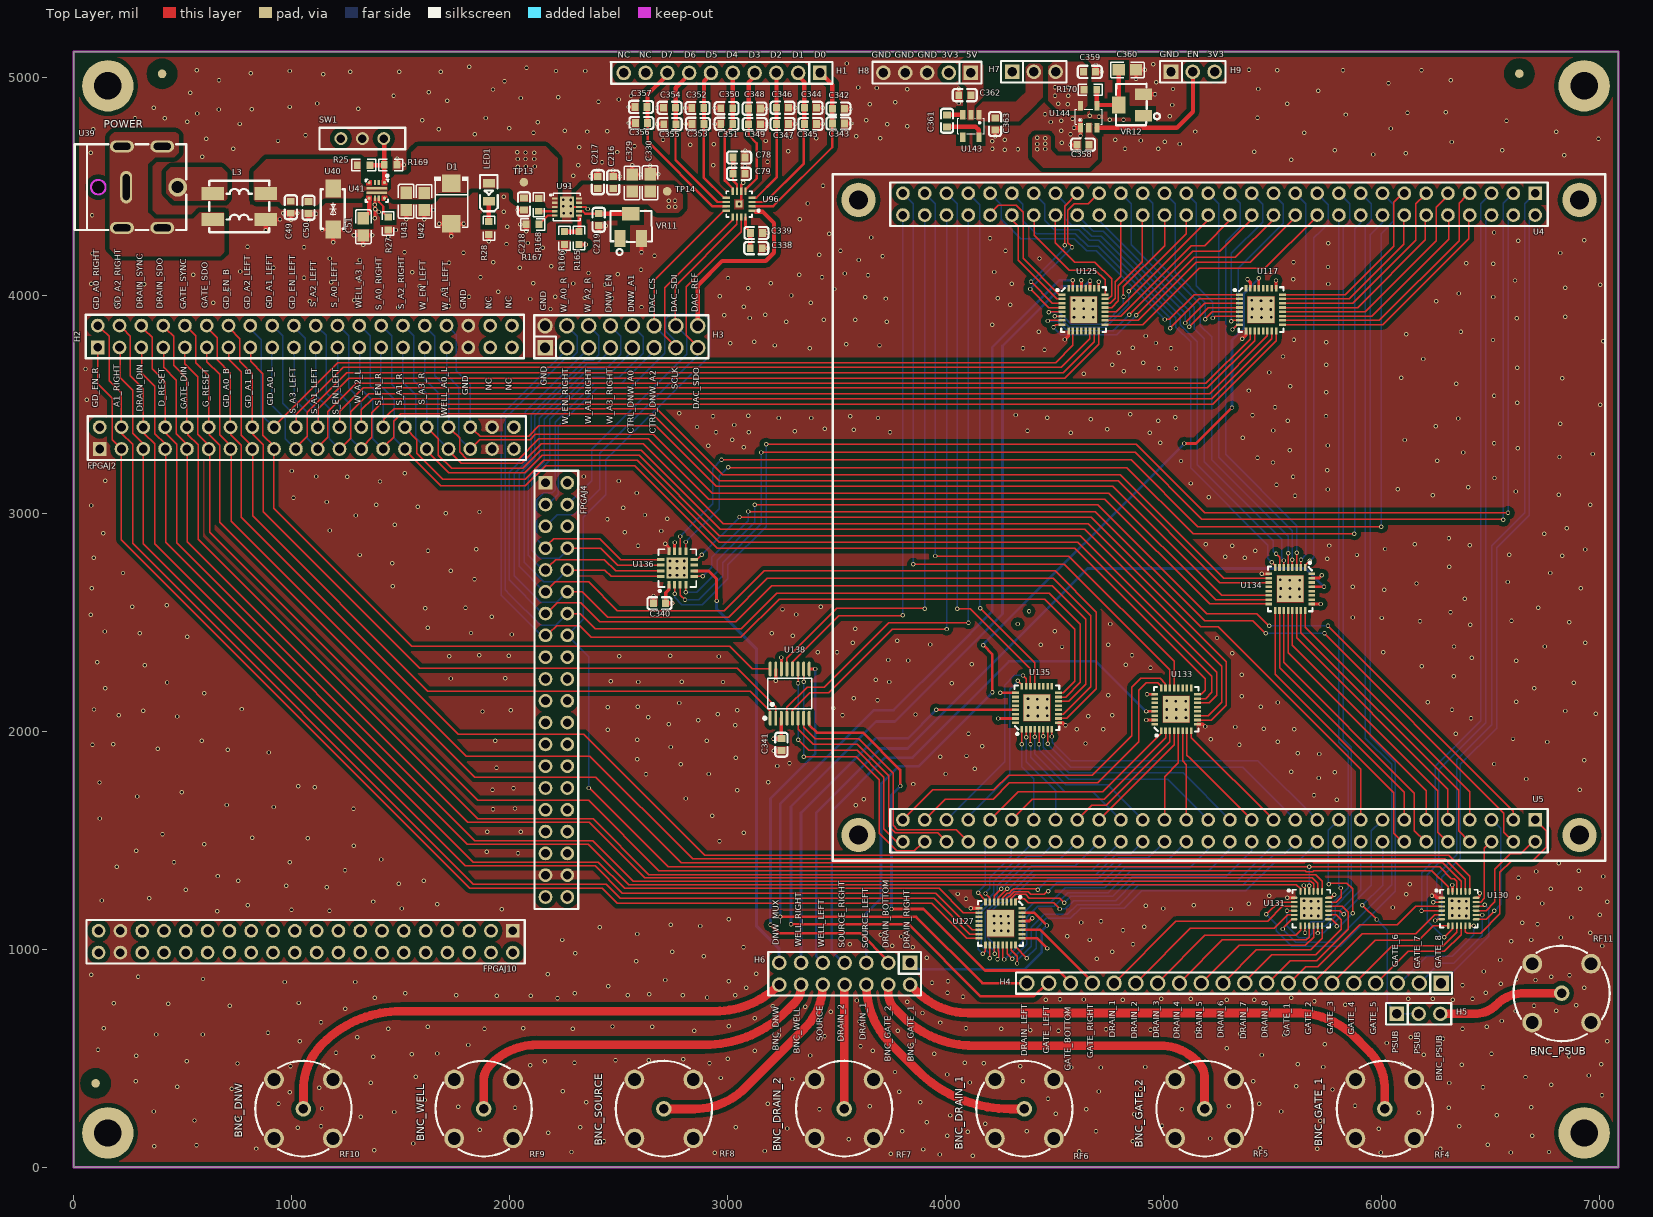
[diagram p0: Top Layer view]
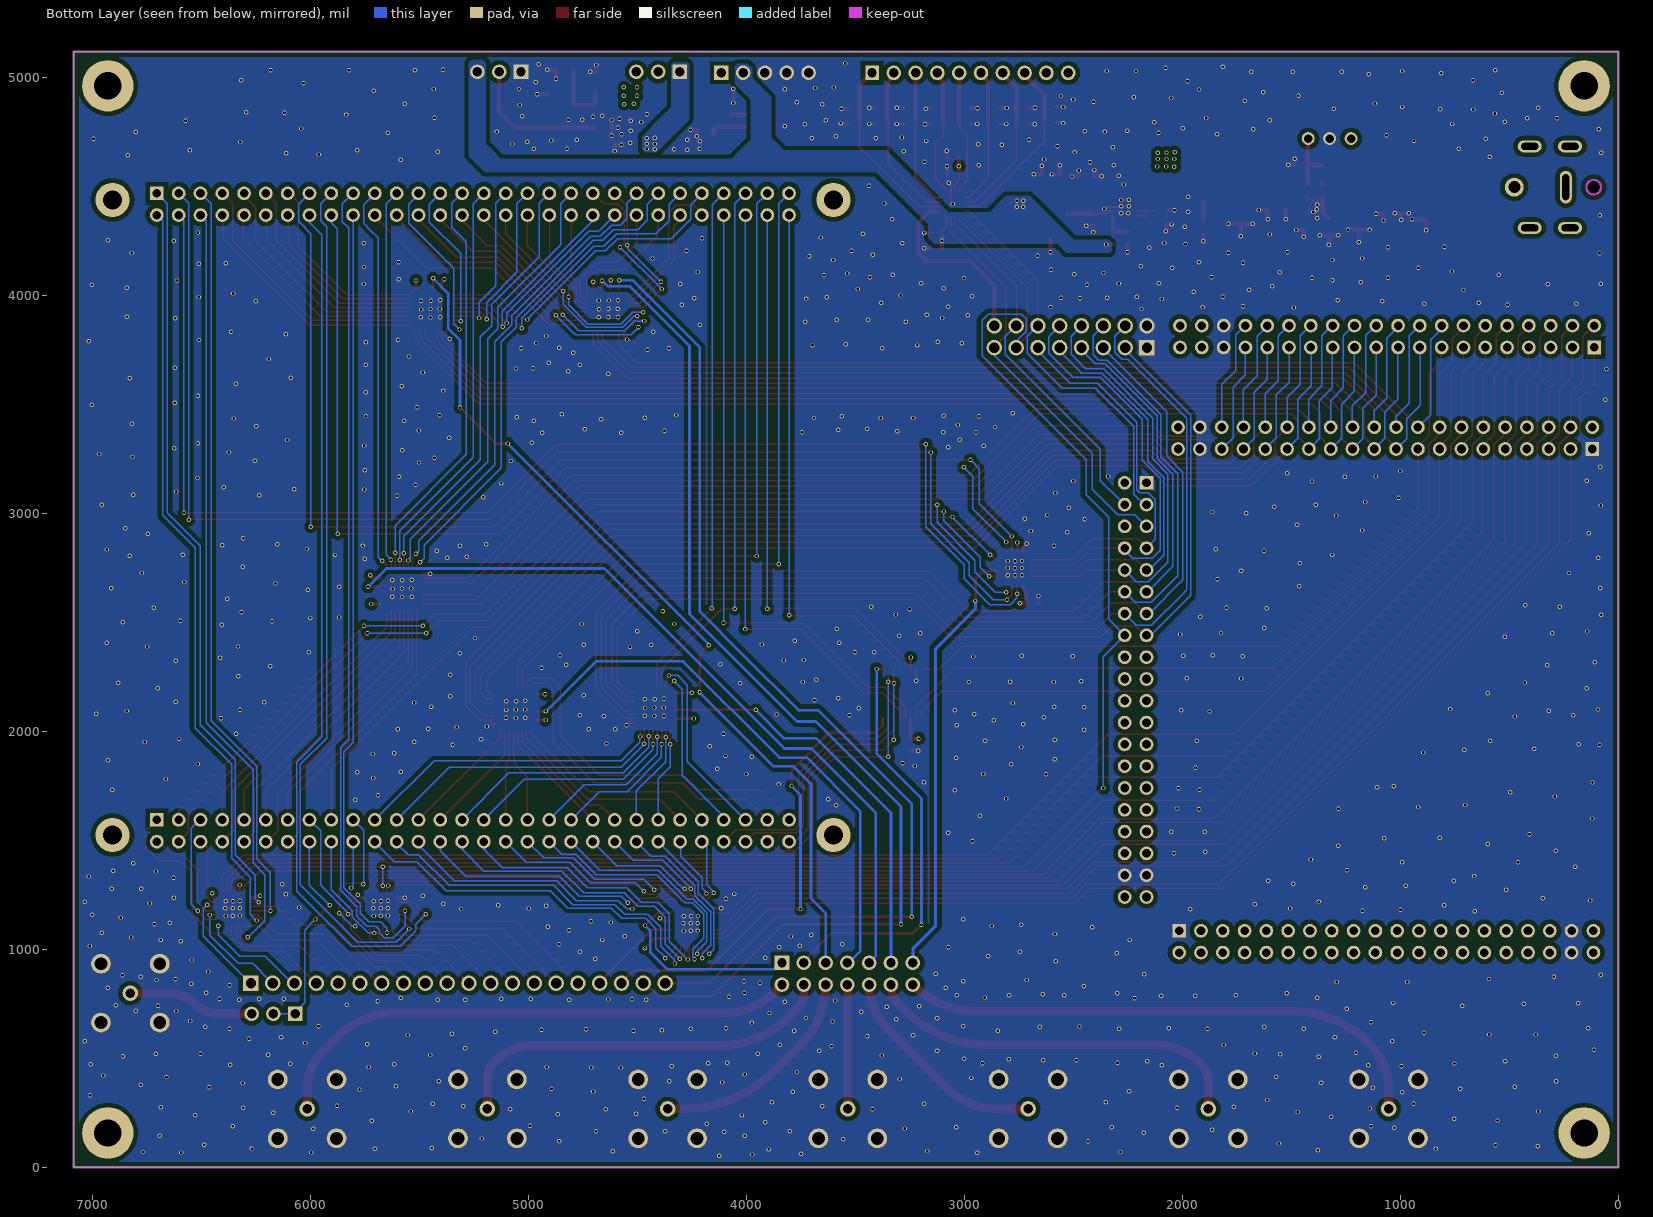
[diagram p1: Bottom Layer view, seen from below]
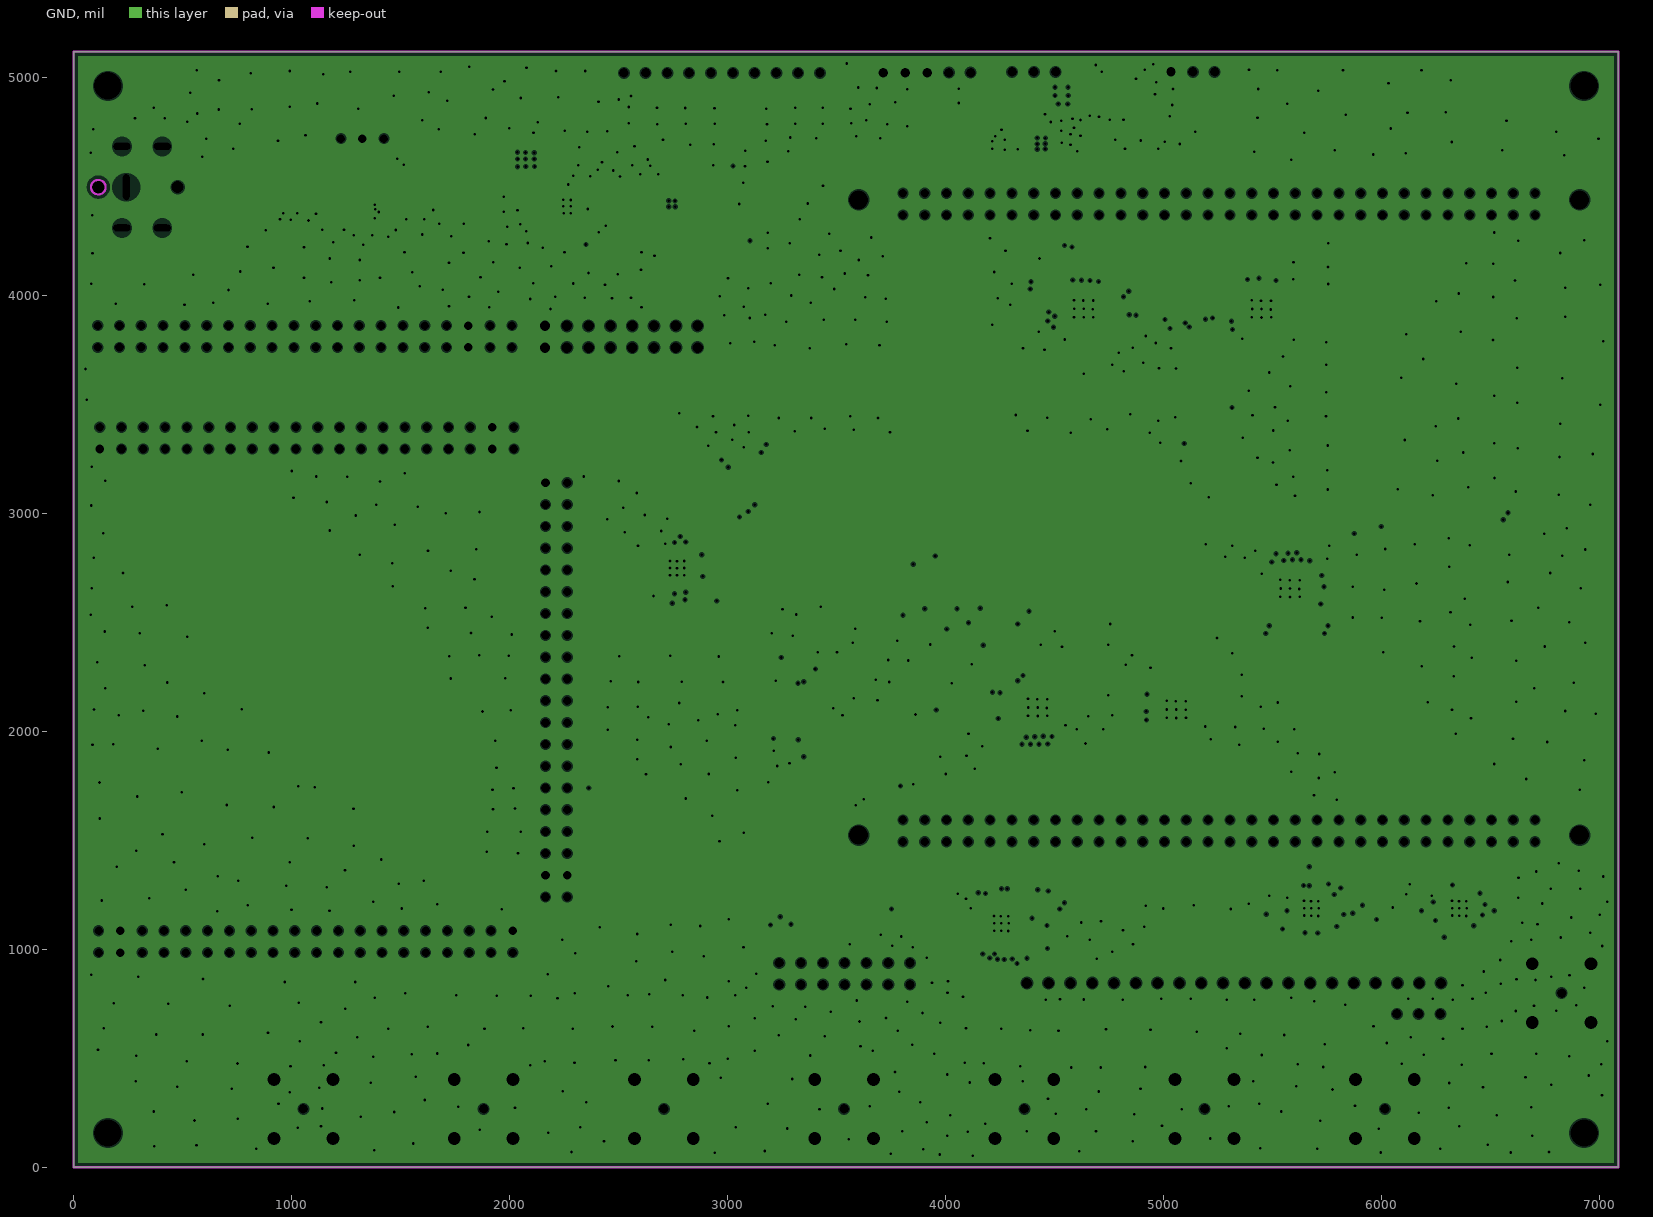
[diagram p2: GND, clearances drawn from the general rule]
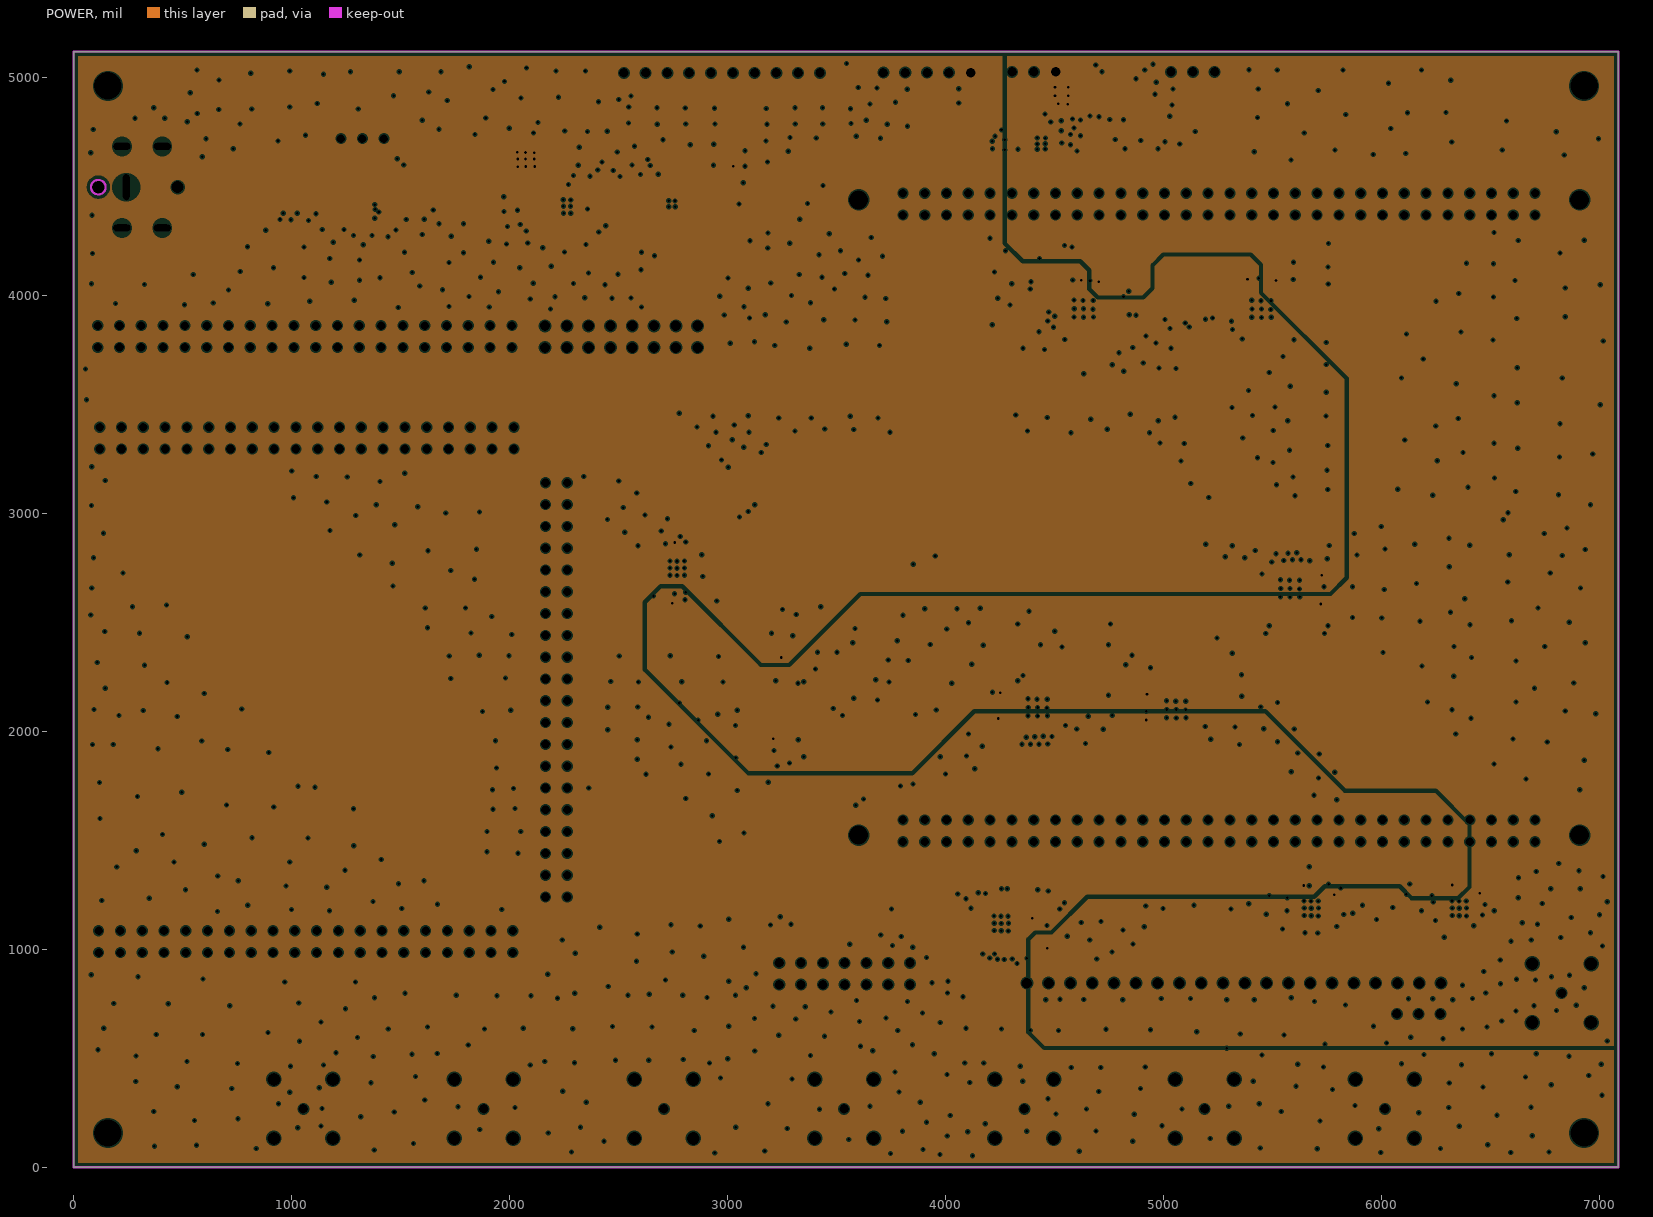
[diagram p3: POWER, clearances drawn from the general rule]
# Altium PCB MISC82799.PcbDoc (part 1 of 5)
Units mil, origin at the board's own origin, x right, y up, seen from the top; angles counter-clockwise.
Board outline 7086.61 x 5118.11 mil, 4 copper layers (Top Layer, GND, POWER, Bottom Layer); 95 components, 232 nets, 857 pads, 1291 vias.

## Layer stack, top to bottom (the 12.6 mil dielectric is the usual default, probably not edited)
Top Layer: signal copper 1.4
Dielectric: core 12.6, FR-4, Dk 4.8
GND: plane copper 1.4, net GND
Dielectric: prepreg 12.6, FR-4, Dk 4.8
POWER: plane copper 1.4, net (Multiple Nets)
Dielectric: core 12.6, FR-4, Dk 4.8
Bottom Layer: signal copper 1.4

## Board outline
0,0 7086.61,0 7086.61,5118.11 0,5118.11

## Design rules (kind name [scope] priority, off if disabled: settings)
Clearance Clearance_2 [haspad('free-mark')] p1: gap=50
Clearance Clearance_1 [inpolygon] p2: gap=6
Clearance [All] p3: gap=6
DiffPairsRouting [All] p1: maxlimit=6 minlimit=6 mostfreqgap=6 maxuncoupledlength=500
HoleSize [All] p1: absolutevalues=TRUE maxlimit=500 minlimit=1 maxpercent=80.000 minpercent=20.000
HoleToHoleClearance [All] p1: gap=0 allowstackedmicrovias=TRUE
MinimumSolderMaskSliver [All] p1: minsoldermaskwidth=0
PlaneClearance [All] p1: clearance=6
PlaneConnect [All] p1: planeconnectstyle=Direct reliefexpansion=20 reliefentries=4 reliefconductorwidth=10 reliefairgap=10
PolygonConnect [All] p1: connectstyle=Direct reliefconductorwidth=10 reliefentries=4 polygonreliefangle="90 Angle"
RoutingVias [All] p1: holewidth=12 width=20 viastyle="Through Hole" minholewidth=12 minwidth=20 maxholewidth=12 maxwidth=20
SilkToSilkClearance [All] p1: silktosilkclearance=0
SilkscreenOverComponentPads [All] p1: minsilkscreentomaskgap=0
SolderMaskExpansion [All] p1: expansion=4
Width [All] p1: maxlimit=40 minlimit=6 preferedwidth=6
20 further rules are at their usual default settings.

## Classes and differential pairs
component class 2_MUX: H4 H5 H6 RF4 RF5 RF6 RF7 RF8 RF9 RF10 RF11 U117 U125 U127 U130 U131 U133 U134 U135 U136 U138
component class 1_Power: C49 C50 C51 C78 C79 C216 C217 C218 C219 C329 C330 C338 C339 C340 C341 C342 C343 C344 C345 C346 C347 C348 C349 C350 C351 C352 C353 C354 C355 C356 C357 C358 C359 C360 C361 C362 C363 D1 FPGAJ2 FPGAJ4 FPGAJ10 H1 H2 H3 H7 H8 H9 L3 LED1 R25 R27 R28 R165 R166 R167 R168 R169 R170 SW1 TP13 TP14 U4 U5 U39 U40 U41 U42 U43 U91 U96 U143 U144 VR11 VR12

## Components (designator, comment, footprint, x,y, rotation, side; value= is the part's Value field where it differs from the comment)
C49 "100nF" C0603 997,4404 r90 top
C50 "100nF" C0603 1078,4402 r90 top
C51 "10nF" C0805 1329,4314 r90 top
C78 "100nF" C0603 3053,4632 r180 top
C79 "10uF" C0603 3052.24,4557.36 r180 top
C216 "22uF" C0603 2475.61,4517.13 r270 top
C217 "22uF" C0603 2405,4518 r270 top
C218 "22uF" C0603 2066,4418 r90 top
C219 "4.7uF" C0603 2409,4347 r90 top
C329 "100nF" C0805 2562.12,4515 r270 top
C330 "10uF" C0805 2645,4516 r270 top
C338 "100nF" C0603 3131.5,4216.36 r180 top
C339 "10uF" C0603 3132,4286 r180 top
C340 "100nF" C0603 2688,2587 r0 top
C341 "10uF" C0603 3247,1939 r90 top
C342 "100nF" C0603 3508.15,4856 r180 top
C343 "10uF" C0603 3508.39,4788.31 r180 top
C344 "100nF" C0603 3380.15,4860 r180 top
C345 "10uF" C0603 3380.15,4786 r180 top
C346 "100nF" C0603 3252.16,4860.31 r180 top
C347 "10uF" C0603 3252.15,4786 r180 top
C348 "100nF" C0603 3123.67,4856.31 r180 top
C349 "10uF" C0603 3124.15,4785 r180 top
C350 "100nF" C0603 2996.15,4858 r0 top
C351 "10uF" C0603 2996.15,4786 r0 top
C352 "100nF" C0603 2863.15,4859 r0 top
C353 "10uF" C0603 2864.15,4786 r0 top
C354 "100nF" C0603 2734.15,4859.89 r0 top
C355 "10uF" C0603 2735.15,4785 r0 top
C356 "100nF" C0603 2605.15,4790 r0 top
C357 "10uF" C0603 2603.39,4863.89 r0 top
C358 "2.2uF" C0603 4631,4691 r0 top
C359 "2.2uF" C0603 4661,5025 r180 top
C360 "10nF" C0805 4834,5034 r180 top
C361 "1uF" C0603 4006.33,4800.13 r270 top
C362 "1uF" C0603 4088.33,4918.13 r0 top
C363 "1uF" C0603 4227.33,4786.13 r90 top
D1 "VS-10BQ015HM3/5BT" SMB_L4.6-W3.6-LS5.3-RD 1733,4421 r270 top
FPGAJ2 "2.54-2*20" HDR-TH_40P-P2.54-V-F-R2-C20-S2.54 1070,3345 r0 top
FPGAJ4 "2.54-2*20" HDR-TH_40P-P2.54-V-F-R2-C20-S2.54 2215,2190 r270 top
FPGAJ10 "2.54-2*20" HDR-TH_40P-P2.54-V-F-R2-C20-S2.54 1065,1035 r180 top
H1 "PZ254V-11-10P" HDR-TH_10P-P2.54-V-M 2974,5020 r180 top
H2 "PZ254-2-20-W-8.5" HDR-TH_40P-P2.54-V-F-R2-C20-S2.54 1061,3811 r0 top
H3 "PZ254V-12-16P" HDR-TH_16P-P2.54-V-M-R2-C8-S2.54 2513,3810 r0 top
H4 "PZ254-1-20-W-8.5" HDR-TH_20P-P2.54-V-M-1 5323,845 r180 top
H5 "PZ254V-11-03P" HDR-TH_3P-P2.54-V-M 6170,704 r0 top
H6 "PZ254V-12-14P" HDR-TH_14P-P2.54-V-M-R2-C7-S2.54 3537,888 r180 top
H7 "PZ254V-11-03P" HDR-TH_3P-P2.54-V-M 4405,5025 r0 top
H8 "PZ254V-11-05P" HDR-TH_5P-P2.54-V-M 3915,5021 r180 top
H9 "PZ254V-11-03P" HDR-TH_3P-P2.54-V-M 5134,5025 r0 top
L3 "PCAQ7060MW-301" FILTER-SMD_4P-L7.0-W6.0-BL 760,4407 r270 top
LED1 "NCD0805G1" LED0805-R-RD 1905,4473 r90 top
R25 "" R0603 1331,4597 r0 top
R27 "" R0603 1443,4329 r270 top
R28 "" R0603 1905,4308 r90 top
R165 "" R0603 2318.61,4262.42 r270 top
R166 "" R0603 2252,4262 r90 top
R167 "" R0603 2106,4325 r0 top
R168 "" R0603 2134,4415 r90 top
R169 "" R0603 1455,4598 r0 top
R170 "" R0603 4664,4943 r180 top
RF4 "DOSIN-801-0057" ANT-TH_DOSIN-801-0057 6015,268 r180 top
RF5 "DOSIN-801-0057" ANT-TH_DOSIN-801-0057 5188.23,268 r180 top
RF6 "DOSIN-801-0057" ANT-TH_DOSIN-801-0057 4361.46,268 r180 top
RF7 "DOSIN-801-0057" ANT-TH_DOSIN-801-0057 3534.68,268 r180 top
RF8 "DOSIN-801-0057" ANT-TH_DOSIN-801-0057 2707.91,268 r180 top
RF9 "DOSIN-801-0057" ANT-TH_DOSIN-801-0057 1881.14,268 r180 top
RF10 "DOSIN-801-0057" ANT-TH_DOSIN-801-0057 1054.37,268 r180 top
RF11 "DOSIN-801-0057" ANT-TH_DOSIN-801-0057 6826,799 r0 top
SW1 "K3-1204D" SW-TH_K3-1204D 1325,4719 r0 top
TP13 "5V" Test-Point-0.5mm 2066,4519 r90 top
TP14 "3P3V" Test-Point-0.5mm 2723,4477 r90 top
U4 "ZX-PM2.54-2-30PY" HDR-TH_60P-P2.54-V-F-R2-C30-S2.54 5254.35,4417.81 r180 top locked
U5 "ZX-PM2.54-2-30PY" HDR-TH_60P-P2.54-V-F-R2-C30-S2.54 5254.35,1543.8 r180 top locked
U39 "HX DC007B-2.5" DC-IN-TH_HX-DC007B-2.5 350,4496 r0 top
U40 "SMAJ12CA" SMA_L4.3-W2.7-LS5.1-BI 1191,4396 r90 top
U41 "TPS259472ARPWR" VQFN-10_L2.0-W2.0-P0.45-TL 1391,4481 r270 top
U42 "22uF" C0805 1608.25,4430.56 r90 top
U43 "22uF" C0805 1526,4431 r90 top
U91 "LT3045IDD#PBF" DFN-10_L3.0-W3.0-P0.50-BL-EP-3 2263,4405 r270 top
U96 "DAC80508ZRTER" WQFN-16_L3.0-W3.0-P0.50-TL-EP0.8 3053,4418 r180 top
U117 "ADG1406BCPZ-REEL7" LFCSP-32_L5.0-W5.0-P0.50-TL-EP3.1 5447,3934 r0 top
U125 "ADG1407BCPZ-REEL7" LFCSP-32_L5.0-W5.0-P0.50-BL-EP3.1 4633,3934 r270 top locked
U127 "ADG1407BCPZ-REEL7" LFCSP-32_L5.0-W5.0-P0.50-BL-EP3.1 4252,1119 r180 top
U130 "ADG1414BCPZ-REEL7" LFCSP-24_L4.0-W4.0-P0.50-BL-EP 6355,1187 r270 top locked
U131 "ADG1414BCPZ-REEL7" LFCSP-24_L4.0-W4.0-P0.50-BL-EP 5678,1187 r270 top
U133 "ADG1406BCPZ-REEL7" LFCSP-32_L5.0-W5.0-P0.50-TL-EP3.1 5058,2101 r90 top
U134 "ADG1406BCPZ-REEL7" LFCSP-32_L5.0-W5.0-P0.50-TL-EP3.1 5581,2653 r270 top
U135 "ADG1406BCPZ-REEL7" LFCSP-32_L5.0-W5.0-P0.50-TL-EP3.1 4419,2108 r90 top
U136 "ADG1408YCPZ-REEL7" LFCSP-16_L4.0-W4.0-P0.65-BL-EP 2770,2749 r0 top
U138 "ADG1409YRUZ-REEL7" TSSOP-16_L5.0-W4.4-P0.65-LS6.4-BL 3285,2173 r0 top
U143 "TPS60403DBVR" SOT-23-5_L3.0-W1.7-P0.95-LS2.8-BR 4116.12,4776.13 r90 top
U144 "TPS72301DBVR" SOT-23-5_L3.0-W1.7-P0.95-LS2.8-BR 4656.56,4819 r270 top
VR11 "" RES-ADJ-SMD_3224W 2556,4317 r0 top
VR12 "" RES-ADJ-SMD_3224W 4851,4873 r90 top

## Footprints (in the part's own frame and the unit in brackets; to place one, negate y for a bottom-side part, rotate by r counter-clockwise, add the part's x,y. Pads: shape width x height; smd on the part's side, far side on the other; paste and mask are expansions set on the pad)
ANT-TH_DOSIN-801-0057 [mm]
  round 1.8 hole 1.1: 1(0,0)
  round 2.3 hole 1.5: 2(-3.429,3.429) 3(3.429,3.429) 4(3.429,-3.429) 5(-3.429,-3.429)
  silkscreen extent -5.6,-5.6 5.6,5.53
C0603 [mm]
  rect 0.8x0.9 smd: 1(-0.7,0) 2(0.7,0)
  silkscreen extent -1.41,-0.71 1.39,0.72
C0805 [mm]
  rect 1.41x1.35 smd paste-100 mask+0.051: 1(-1,0) 2(1,0)
  silkscreen extent -1.96,-0.9 1.96,0.9
DC-IN-TH_HX-DC007B-2.5 [mm]
  round 2.2 hole 1.4: 1(3.25,0)
  oval 1.4x3.8 hole 0.8 slot 3 at 90 deg: 2(-2.75,0)
  oval 2.8x1.4 hole 0.8 slot 2 at 0 deg: 3(-3.25,-4.75) 3(-3.25,4.75) 3(1.45,-4.75) 3(1.45,4.75)
  Keep-Out Layer circle w0.005: c-6,0 r0.85
  Keep-Out Layer board cut-out: -5.15,0 -5.234,0.369 -5.47,0.664 -5.811,0.829 -6.189,0.829 -6.53,0.664 -6.766,0.369 -6.85,0 -6.85,0 -6.766,-0.369 -6.53,-0.665 -6.189,-0.829 -5.811,-0.829 -5.47,-0.665 -5.234,-0.369 -5.15,0
  Keep-Out Layer circle w0.254: c-6,0 r0.85
  silkscreen extent -8.75,-5 4.25,5
DFN-10_L3.0-W3.0-P0.50-BL-EP-3 [mm]
  rect 0.25x0.65 smd: 1(-1,-1.411) 2(-0.5,-1.411) 3(0,-1.411) 4(0.5,-1.411) 5(1,-1.411) 6(1,1.411) 7(0.5,1.411) 8(0,1.411) 9(-0.5,1.411) 10(-1,1.411)
  rect 2.5x1.6 smd: 11(0,0)
  silkscreen extent -1.58,-2 1.58,1.58
FILTER-SMD_4P-L7.0-W6.0-BL [mm]
  rect 1.501x2.6 smd: 1(-1.5,-3.1) 2(1.5,-3.1) 3(1.5,3.1) 4(-1.5,3.1)
  silkscreen extent -3,-3.5 3,3.5
HDR-TH_3P-P2.54-V-M [mm]
  rect 1.7x1.7 hole 1.1: 1(-2.54,0)
  round 1.7 hole 1.1: 2(0,0) 3(2.54,0)
  silkscreen extent -3.81,-1.25 3.81,1.25
HDR-TH_5P-P2.54-V-M [mm]
  rect 1.7x1.7 hole 1.1: 1(-5.08,0)
  round 1.7 hole 1.1: 2(-2.54,0) 3(0,0) 4(2.54,0) 5(5.08,0)
  silkscreen extent -6.35,-1.27 6.35,1.27
HDR-TH_10P-P2.54-V-M [mm]
  rect 1.575x1.7 hole 1.1: 1(-11.43,0)
  round 1.7 hole 1.1: 2(-8.89,0) 3(-6.35,0) 4(-3.81,0) 5(-1.27,0) 6(1.27,0) 7(3.81,0) 8(6.35,0) 9(8.89,0) 10(11.43,0)
  silkscreen extent -12.9,-1.27 12.95,1.27
HDR-TH_14P-P2.54-V-M-R2-C7-S2.54 [mm]
  rect 1.7x1.7 hole 1.1: 1(-7.62,-1.27)
  round 1.7 hole 1.1: 2(-7.62,1.27) 3(-5.08,-1.27) 4(-5.08,1.27) 5(-2.54,-1.27) 6(-2.54,1.27) 7(0,-1.27) 8(0,1.27) 9(2.54,-1.27) 10(2.54,1.27) 11(5.08,-1.27) 12(5.08,1.27) 13(7.62,-1.27) 14(7.62,1.27)
  silkscreen extent -8.89,-2.54 8.89,2.54
HDR-TH_16P-P2.54-V-M-R2-C8-S2.54 [mm]
  rect 1.8x1.8 hole 1.2: 1(-8.89,-1.27)
  round 1.8 hole 1.2: 2(-8.89,1.27) 3(-6.35,-1.27) 4(-6.35,1.27) 5(-3.81,-1.27) 6(-3.81,1.27) 7(-1.27,-1.27) 8(-1.27,1.27) 9(1.27,-1.27) 10(1.27,1.27) 11(3.81,-1.27) 12(3.81,1.27) 13(6.35,-1.27) 14(6.35,1.27) 15(8.89,-1.27) 16(8.89,1.27)
  silkscreen extent -10.16,-2.5 10.16,2.5
HDR-TH_20P-P2.54-V-M-1 [mm]
  rect 1.8x1.8 hole 1.2: 1(-24.13,0)
  round 1.8 hole 1.2: 2(-21.59,0) 3(-19.05,0) 4(-16.51,0) 5(-13.97,0) 6(-11.43,0) 7(-8.89,0) 8(-6.35,0) 9(-3.81,0) 10(-1.27,0) 11(1.27,0) 12(3.81,0) 13(6.35,0) 14(8.89,0) 15(11.43,0) 16(13.97,0) 17(16.51,0) 18(19.05,0) 19(21.59,0) 20(24.13,0)
  silkscreen extent -25.4,-1.25 25.4,1.25
HDR-TH_40P-P2.54-V-F-R2-C20-S2.54 [mm]
  rect 1.6x1.6 hole 1: 1(-24.13,-1.27)
  round 1.6 hole 1: 2(-24.13,1.27) 3(-21.59,-1.27) 4(-21.59,1.27) 5(-19.05,-1.27) 6(-19.05,1.27) 7(-16.51,-1.27) 8(-16.51,1.27) 9(-13.97,-1.27) 10(-13.97,1.27) 11(-11.43,-1.27) 12(-11.43,1.27) 13(-8.89,-1.27) 14(-8.89,1.27) 15(-6.35,-1.27) 16(-6.35,1.27) 17(-3.81,-1.27) 18(-3.81,1.27) 19(-1.27,-1.27) 20(-1.27,1.27) 21(1.27,-1.27) 22(1.27,1.27) 23(3.81,-1.27) 24(3.81,1.27) 25(6.35,-1.27) 26(6.35,1.27) 27(8.89,-1.27) 28(8.89,1.27) 29(11.43,-1.27) 30(11.43,1.27) 31(13.97,-1.27) 32(13.97,1.27) 33(16.51,-1.27) 34(16.51,1.27) 35(19.05,-1.27) 36(19.05,1.27) 37(21.59,-1.27) 38(21.59,1.27) 39(24.13,-1.27) 40(24.13,1.27)
  silkscreen extent -25.53,-2.54 25.53,2.54
HDR-TH_60P-P2.54-V-F-R2-C30-S2.54 [mm]
  rect 1.6x1.6 hole 1: 1(-36.83,-1.27)
  round 1.6 hole 1: 2(-36.83,1.27) 3(-34.29,-1.27) 4(-34.29,1.27) 5(-31.75,-1.27) 6(-31.75,1.27) 7(-29.21,-1.27) 8(-29.21,1.27) 9(-26.67,-1.27) 10(-26.67,1.27) 11(-24.13,-1.27) 12(-24.13,1.27) 13(-21.59,-1.27) 14(-21.59,1.27) 15(-19.05,-1.27) 16(-19.05,1.27) 17(-16.51,-1.27) 18(-16.51,1.27) 19(-13.97,-1.27) 20(-13.97,1.27) 21(-11.43,-1.27) 22(-11.43,1.27) 23(-8.89,-1.27) 24(-8.89,1.27) 25(-6.35,-1.27) 26(-6.35,1.27) 27(-3.81,-1.27) 28(-3.81,1.27) 29(-1.27,-1.27) 30(-1.27,1.27) 31(1.27,-1.27) 32(1.27,1.27) 33(3.81,-1.27) 34(3.81,1.27) 35(6.35,-1.27) 36(6.35,1.27) 37(8.89,-1.27) 38(8.89,1.27) 39(11.43,-1.27) 40(11.43,1.27) 41(13.97,-1.27) 42(13.97,1.27) 43(16.51,-1.27) 44(16.51,1.27) 45(19.05,-1.27) 46(19.05,1.27) 47(21.59,-1.27) 48(21.59,1.27) 49(24.13,-1.27) 50(24.13,1.27) 51(26.67,-1.27) 52(26.67,1.27) 53(29.21,-1.27) 54(29.21,1.27) 55(31.75,-1.27) 56(31.75,1.27) 57(34.29,-1.27) 58(34.29,1.27) 59(36.83,-1.27) 60(36.83,1.27)
  silkscreen extent -38.3,-2.54 38.3,2.54
LED0805-R-RD [mm]
  rect 1x1.4 smd: 1(1.05,0) 2(-1.05,0)
  silkscreen extent -2.22,-1.04 1.99,1.01
LFCSP-16_L4.0-W4.0-P0.65-BL-EP [mm]
  rect 0.35x0.9 smd: 1(-0.975,-1.95) 2(-0.325,-1.95) 3(0.325,-1.95) 4(0.975,-1.95) 9(0.975,1.95) 10(0.325,1.95) 11(-0.325,1.95) 12(-0.975,1.95)
  rect 0.9x0.35 smd: 5(1.95,-0.975) 6(1.95,-0.325) 7(1.95,0.325) 8(1.95,0.975) 13(-1.95,0.975) 14(-1.95,0.325) 15(-1.95,-0.325) 16(-1.95,-0.975)
  rect 2.5x2.5 smd: 17(0,0)
  silkscreen extent -2.2,-2.8 2.2,2.2
LFCSP-24_L4.0-W4.0-P0.50-BL-EP [mm]
  oval 0.25x0.8 smd paste-100 mask+0.051: 1(-1.25,-2) 2(-0.749,-2) 3(-0.249,-2) 4(0.249,-2) 5(0.749,-2) 6(1.25,-2) 13(1.25,2) 14(0.749,2) 15(0.249,2) 16(-0.249,2) 17(-0.749,2) 18(-1.25,2)
  oval 0.8x0.25 smd paste-100 mask+0.051: 7(2,-1.25) 8(2,-0.749) 9(2,-0.249) 10(2,0.249) 11(2,0.749) 12(2,1.25) 19(-2,1.25) 20(-2,0.749) 21(-2,0.249) 22(-2,-0.249) 23(-2,-0.749) 24(-2,-1.25)
  rect 2.6x2.6 smd paste-100 mask+0.051: 25(0,0)
  silkscreen extent -2.22,-2.75 2.2,2.2
LFCSP-32_L5.0-W5.0-P0.50-BL-EP3.1 [mm]
  rect 0.3x0.8 smd paste-100 mask+0.051: 1(-1.75,-2.5) 2(-1.25,-2.5) 3(-0.75,-2.5) 4(-0.25,-2.5) 5(0.25,-2.5) 6(0.75,-2.5) 7(1.25,-2.5) 8(1.75,-2.5) 17(1.75,2.5) 18(1.25,2.5) 19(0.75,2.5) 20(0.25,2.5) 21(-0.25,2.5) 22(-0.75,2.5) 23(-1.25,2.5) 24(-1.75,2.5)
  rect 0.8x0.3 smd paste-100 mask+0.051: 9(2.5,-1.75) 10(2.5,-1.25) 11(2.5,-0.75) 12(2.5,-0.25) 13(2.5,0.25) 14(2.5,0.75) 15(2.5,1.25) 16(2.5,1.75) 25(-2.5,1.75) 26(-2.5,1.25) 27(-2.5,0.75) 28(-2.5,0.25) 29(-2.5,-0.25) 30(-2.5,-0.75) 31(-2.5,-1.25) 32(-2.5,-1.75)
  rect 3.1x3.1 smd paste-100 mask+0.051: 33(0,0)
  silkscreen extent -2.6,-3.17 2.6,2.6
LFCSP-32_L5.0-W5.0-P0.50-TL-EP3.1 [mm]
  rect 0.8x0.3 smd paste-100 mask+0.05: 1(-2.5,1.75) 2(-2.5,1.25) 3(-2.5,0.75) 4(-2.5,0.25) 5(-2.5,-0.25) 6(-2.5,-0.75) 7(-2.5,-1.25) 8(-2.5,-1.75) 17(2.5,-1.75) 18(2.5,-1.25) 19(2.5,-0.75) 20(2.5,-0.25) 21(2.5,0.25) 22(2.5,0.75) 23(2.5,1.25) 24(2.5,1.75)
  rect 0.3x0.8 smd paste-100 mask+0.05: 9(-1.75,-2.5) 10(-1.25,-2.5) 11(-0.75,-2.5) 12(-0.25,-2.5) 13(0.25,-2.5) 14(0.75,-2.5) 15(1.25,-2.5) 16(1.75,-2.5) 25(1.75,2.5) 26(1.25,2.5) 27(0.75,2.5) 28(0.25,2.5) 29(-0.25,2.5) 30(-0.75,2.5) 31(-1.25,2.5) 32(-1.75,2.5)
  rect 3.1x3.1 smd paste-100 mask+0.05: 33(0,0)
  silkscreen extent -3.17,-2.6 2.6,2.6
R0603 [mil]
  rect 31.75x34.02 smd paste-3937.01 mask+2: 1(-29.66,0) 2(29.66,0)
  silkscreen extent -55,-26 55,26
RES-ADJ-SMD_3224W [mm]
  rect 1.3x2 smd: 1(-1.25,-1.45) 3(1.25,-1.45)
  rect 2x1.6 smd: 2(0,1.45)
  silkscreen extent -2.36,-3.36 2.47,1.77
SMA_L4.3-W2.7-LS5.1-BI [mm]
  rect 2.1x1.8 smd: 1(-2.4,0) 2(2.4,0)
  silkscreen extent -2.3,-1.35 2.3,1.45
SMB_L4.6-W3.6-LS5.3-RD [mil]
  rect 80.61x86.31 smd: 1(-92.94,0) 2(92.94,0)
  silkscreen extent -123,-77 108,77
SOT-23-5_L3.0-W1.7-P0.95-LS2.8-BR [mm]
  rect 1.1x0.6 smd: 1(1.3,-0.95) 2(1.3,0) 3(1.3,0.95) 4(-1.3,0.95) 5(-1.3,-0.95)
  silkscreen extent -0.9,-1.55 0.9,1.55
SW-TH_K3-1204D [mm]
  round 1.5 hole 1: 1(-2.5,0) 2(0,0) 3(2.5,0)
  silkscreen extent -5,-1.25 5,1.25
Test-Point-0.5mm [mm]
  round 1 smd: 1(0,0)
TSSOP-16_L5.0-W4.4-P0.65-LS6.4-BL [mil]
  oval 13.5x68.17 smd: 1(-89.57,-112.82) 2(-63.98,-112.82) 3(-38.39,-112.82) 4(-12.79,-112.82) 5(12.8,-112.82) 6(38.39,-112.82) 7(63.98,-112.82) 8(89.57,-112.82) 9(89.57,112.82) 10(63.98,112.82) 11(38.39,112.82) 12(12.8,112.82) 13(-12.79,112.82) 14(-38.39,112.82) 15(-63.98,112.82) 16(-89.57,112.82)
  silkscreen extent -120,-119 101,70
VQFN-10_L2.0-W2.0-P0.45-TL [mm]
  round 0.36 smd: 1(-0.915,0.9) 4(-0.905,-0.9) 7(0.915,-0.9) 10(0.915,0.9)
  rect 0.6x0.25 smd paste+0 mask+0.05: 2(-0.905,0.225) 3(-0.905,-0.225) 8(0.905,-0.225) 9(0.905,0.225)
  rect 0.3x2.4 smd paste+0 mask+0.05: 5(-0.235,0) 6(0.265,0)
  Top Layer region: -0.865,1.2 -0.865,0.9 -1.215,0.9 -1.215,0.6 -0.615,0.6 -0.615,0.9 -0.615,0.9 -0.615,1.2
  Top Layer region: -0.855,-1.2 -0.855,-0.9 -1.205,-0.9 -1.205,-0.6 -0.605,-0.6 -0.605,-0.9 -0.605,-0.9 -0.605,-1.2
  Top Layer region: 0.865,-1.2 0.865,-0.9 1.215,-0.9 1.215,-0.6 0.615,-0.6 0.615,-0.9 0.615,-0.9 0.615,-1.2
  Top Layer region: 0.865,1.2 0.865,0.9 1.215,0.9 1.215,0.6 0.615,0.6 0.615,0.9 0.615,0.9 0.615,1.2
  silkscreen extent -1.85,-1.28 1.34,1.36
WQFN-16_L3.0-W3.0-P0.50-TL-EP0.8 [mm]
  rect 0.85x0.28 smd paste+0 mask+0.05: 1(-1.5,0.75) 2(-1.5,0.25) 3(-1.5,-0.25) 4(-1.5,-0.75) 9(1.5,-0.75) 10(1.5,-0.25) 11(1.5,0.25) 12(1.5,0.75)
  rect 0.28x0.85 smd paste+0 mask+0.05: 5(-0.75,-1.5) 6(-0.25,-1.5) 7(0.25,-1.5) 8(0.75,-1.5) 13(0.75,1.5) 14(0.25,1.5) 15(-0.25,1.5) 16(-0.75,1.5)
  rect 0.8x0.8 smd paste+0 mask+0.05: 17(0,0)
  silkscreen extent -2.39,-1.5 1.5,1.5

## Part data
C49 C50: library part CL10B104KA8NNNC
C51 C360: library part CL21B103KBANNNC
C78 C338 C340 C342 C344 C346 C348 C350 C352 C354 C356: library part CL10B104JB8NNNC
C79 C339 C341 C343 C345 C347 C349 C351 C353 C355 C357: library part CL10A106KO8NQNC
C216 C217 C218: library part CL10A226MO7JZNC
C219: library part CL10A475KA8NQNC
C329: library part CL21B104KCFNNNE
C330: library part GRM21BR61H106KE43L
C358 C359: library part CL10A225KB8NNNC
C361 C362 C363: library part CL10A105KB8NNNC
H2: library part PZ254-2-20-W-8.5_C2895000
R25: library part 0603WAF1004T5E
R27: library part RT0603BRD07681RL
R28: library part 0603WAF1001T5E
R165: library part 0603WAF4533T5E
R166: library part AR03BTC5002A
R167: library part 0603WAF2490T5E
R168: library part 0603WAF2003T5E
R169: library part ERJ3RED3573V
R170: library part 0603WAF7502T5E
U42 U43: library part CL21A226KOQNNNE
VR11 VR12: library part 3224W-1-503E

## Free pads (board coordinates)
  round 236.22 hole 125.98: 0(157.48,157.48) 0(157.48,4960.63) 0(6929.13,157.48) 0(6929.13,4960.63)
  round 157.48 hole 86.61: 0(3600.8,1524.11) 0(3600.8,4437.5) 0(6907.89,1524.11) 0(6907.89,4437.5)
  round 39.37 smd mask+39.37: MARK(101,385) MARK(406,5016) MARK(6632,5017)

## Via types
v1: diameter 20, hole 12, Top Layer to Bottom Layer, 1291 vias

## Nets (pads, with @x,y where several pads share a name; then routed paths per layer and width w, separated by ;. In a path a pad name is that pad's centre, name@x,y a point inside that pad or via, vN(x,y) a via of type N, cw(c..) or ccw(c..) an arc to the next point about the centre after c; other vN are vias at no path point)
3P3V: C216.2 C217.2 C329.2 C330.2 C338.2 C339.2 H8.2 H9.3 R165.2 TP14.1 U91.9 U91.10 U96.16 | length 161.9
  Top Layer w12: U96.16@3082.53,4358.94 3082.53,4313.47 C339.2@3101,4295
  Top Layer w20: R165.2@2318.61,4232.76 v1(2350.24,4232.76) ; v1(3103,4250) v1@3103.94,4250 ; C338.2@3103.94,4216.36 v1@3103.94,4250 ; C339.2@3103.94,4274.06 v1@3103.94,4250
  other v1: 2730,4406 2760,4406 2759,4433 2730,4434
5V: C78.2 C79.2 C218.2 C362.2 D1.1 H8.1 LED1.1 R168.2 TP13.1 U41.6 U42.2 U43.2 U91.1 U91.2 U91.3 U96.7 U117.31 U125.29 U127.29 U130.23 U131.23 U133.31 U134.31 U135.31 U136.11 U138.14 U143.2 | length 607.9
  Top Layer w6: v1@5642.2,1287.8 v1(5642.2,1292.75)
  Top Layer w10: v1@5642,1290 5642,1285.88 5648.5,1279.38 U131.23@5648.5,1265.74
  Top Layer w11: C79.2@3025,4546 3025,4527 3043.16,4508.84 U96.7@3043.16,4477.05
  Top Layer w12: v1(6325,1295) 6325.5,1294.5 U130.23@6325.5,1265.74
  Top Layer w14: U136.11@2757.2,2825.77 v1(2757.2,2865.8) ; U138.14@3246.61,2285.82 v1(3246.61,2338.39) ; v1(4241.78,2058.78) U135.31@4320.58,2058.78 ; U127.29@4350.42,1128.85 4382.84,1128.85 v1(4397,1143) ; U125.29@4623.16,4032.42 v1(4623.16,4069.16) ; v1(4921.22,2051.78) U133.31@4959.58,2051.78 ; v1(5385,4073) 5397.78,4060.22 U117.31@5397.78,4032.42 ; U134.31@5679.42,2702.22 5713.22,2702.22 v1(5726,2715)
  Top Layer w20: C79.2@3025.44,4562.56 v1@3025.44,4594 ; v1(3025.44,4592.56) v1@3025.44,4594 ; C78.2@3025.44,4632 v1@3025.44,4594
  Bottom Layer w6: v1@5642.2,1290.2 v1(5642.2,1292.75)
  other v1: 2037,4590 2074,4591 2115,4591 2037,4625 2073,4625 2113,4625 2113,4654 2073,4655 2036,4656
5V_NEG: C340.2 C341.2 C359.2 H7.3 R170.2 U117.25 U125.25 U127.25 U130.18 U131.18 U133.25 U134.25 U135.25 U136.1 U138.3 U144.5 | length 651.4
  Top Layer w12: v1(4250.1,2176.9) U135.25@4320.58,2176.9 ; U127.25@4350.42,1050.1 4420.9,1050.1 v1(4467,1004) ; U125.25@4701.9,4032.42 v1(4701.9,4062.9) ; v1(4924.1,2169.9) U133.25@4959.58,2169.9 ; U117.25@5515.9,4032.42 v1(5515.9,4067.9) ; U134.25@5679.42,2584.1 v1(5721.1,2584.1) ; U131.18@5756.74,1236.2 5768.2,1236.2 v1(5783,1251) ; U130.18@6433.74,1236.2 6441.2,1236.2 6451,1246 v1(6451,1257)
  Top Layer w15: C340.2@2716,2597 2716,2636 2731.61,2651.61 U136.1@2731.61,2672.23 ; C341.2@3246.61,1971.39 U138.3@3246.61,2060.18
  Top Layer w20: C340.2@2715.56,2587 v1(2746,2587) ; v1(3210.44,1966.56) C341.2@3247,1966.56
  other v1: 4561,4877 4517,4878 4502,4916 4563,4916 4502,4954 4562,4954
A_D_C1: U4.16 U131.2 | length 4149.9
  Top Layer w6: v1@5476,1165 5527.5,1216.5 U131.2@5599.26,1216.5
  Bottom Layer w6: v1(5471,1161) 5517,1115 5517,1085 5589,1013 5810,1013 6063,1266 6063,1427 ; U4.16@6004.35,4367.81 6004.35,4334.35 5947,4277 5947,1975 6063,1859 6063,1427 ; 6063,1371 6063,1427
A_D_C2: U4.19 U131.4 | length 3778.9
  Top Layer w6: v1(5566,1177) U131.4@5591,1177
  Bottom Layer w6: v1@5566,1173 5566,1107 5619,1054 5662,1054 5682,1074 5682,1087 5701,1106 5741,1106 5787,1152 5787,1196 5862,1271 5862,1926 5825,1963 5825,4310 5853,4338 5853,4419.16 U4.19@5804.35,4467.81 ; v1(5566,1177) v1@5568,1175
A_D_C3: U4.17 U131.6 | length 3957
  Top Layer w6: v1@5549,1099 5587.8,1137.8 U131.6@5599.26,1137.8
  Bottom Layer w6: v1(5546,1093) 5606,1033 5783,1033 6046,1296 6046,1333 6046,1369 ; U4.17@5904.35,4467.81 5952,4420.16 5952,4341 5925,4314 5925,1969 6046,1848 6046,1369 ; 6046,1365 6046,1369